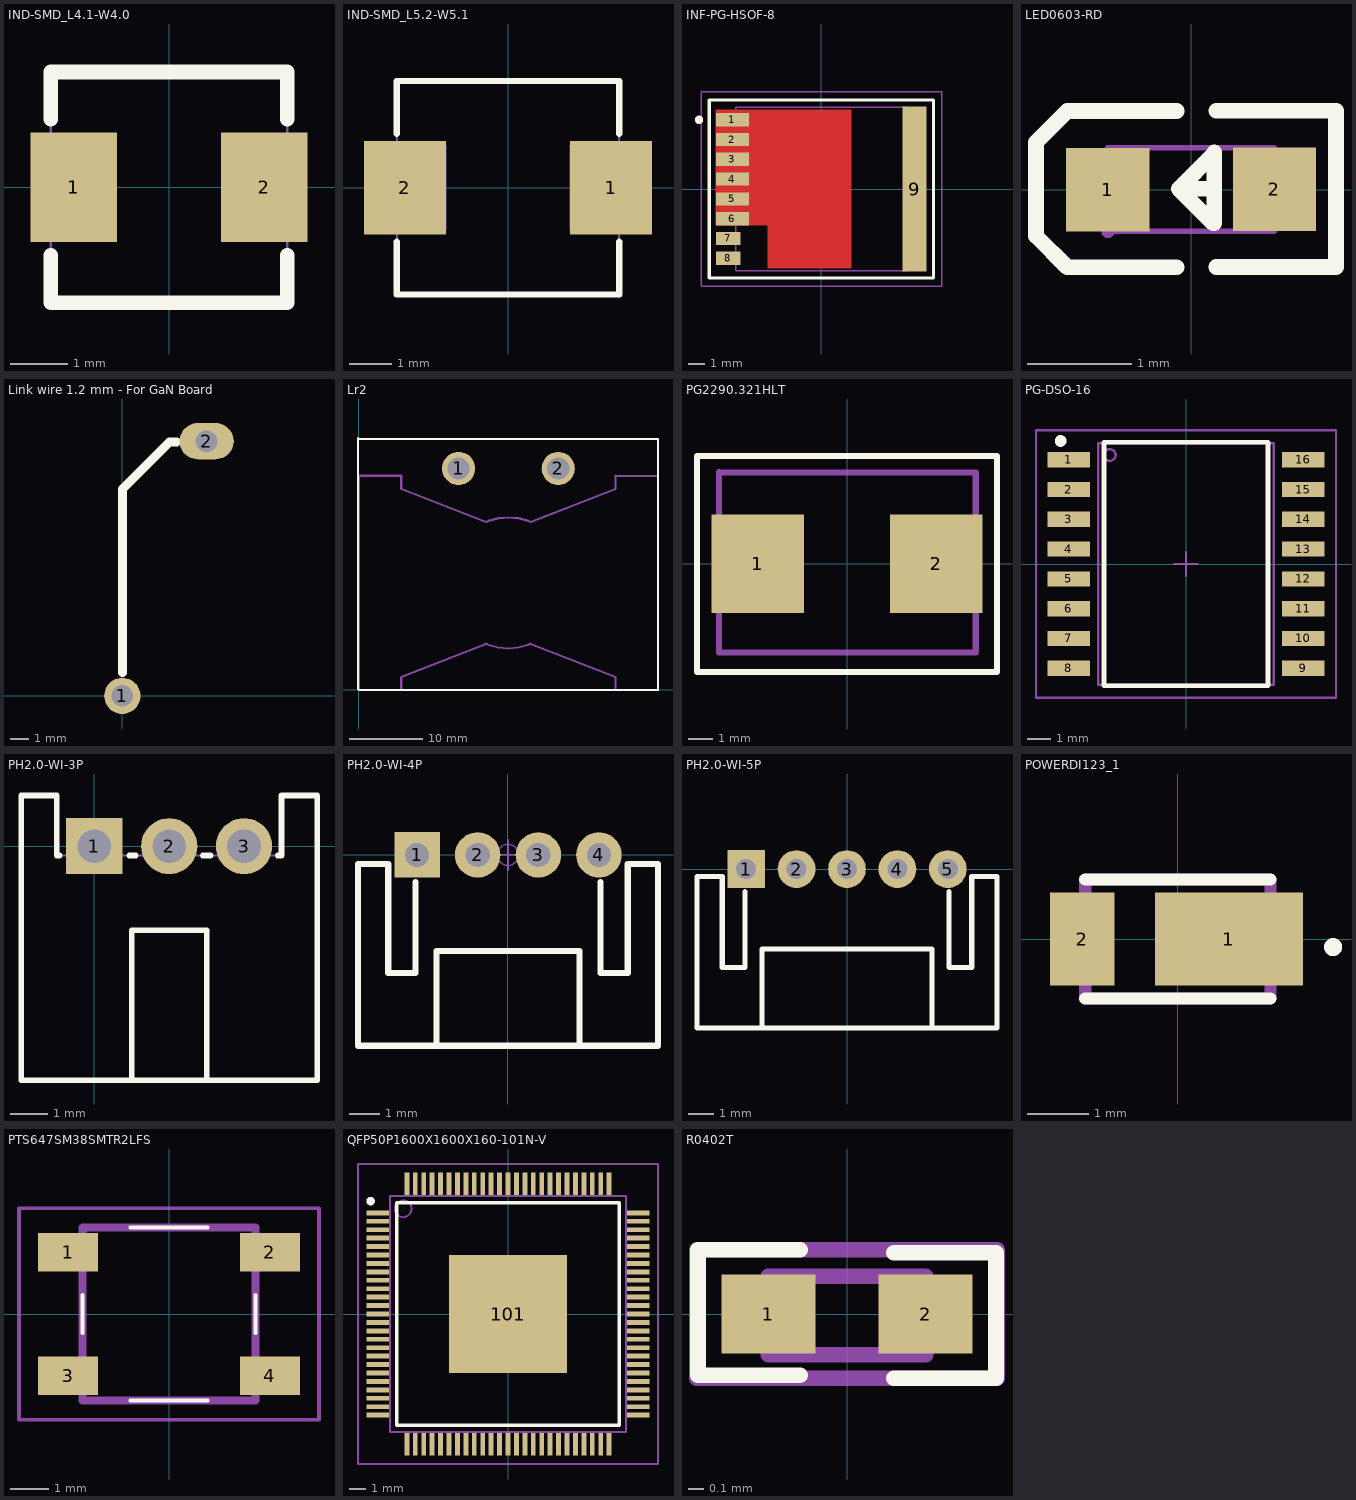
[diagram p0: the footprints below, top view; thin cyan lines are the x and y axes]
# Altium footprint library MISC82254-2.PcbLib: 93 footprints (part 3 of 6)
Each footprint in its own frame and in the unit in brackets; x right, y up, seen from the top. Pads: shape width x height; smd on the part's side, far side on the other; paste and mask are expansions set on the pad; w line width, h text height; cw(c..) or ccw(c..) is an arc to the next point about the centre after c.

## IND-SMD_L4.1-W4.0 [mm]
pads (2):
  rect 1.5x1.9 smd: 1(-1.651,0) 2(1.651,0)
Top Overlay:
  lines w0.254: -2.05,-1.181 -2.05,-2 2.05,-2 2.05,-1.181 ; -2.05,1.181 -2.05,1.999 1.831,1.999 2.05,2 2.05,1.181
Mechanical 15:
  region: -1.99,-2 -1.991,-1.976 -2.026,-1.942 -2.074,-1.942 -2.109,-1.976 -2.11,-2 -2.109,-2.024 -2.074,-2.058 -2.026,-2.058 -1.991,-2.024
  region: -2.05,0.8 -1.05,0.8 -1.05,-0.8 -2.05,-0.8
  region: 1.05,0.8 2.05,0.8 2.05,-0.8 1.05,-0.8
  lines w0.051: -2.05,-2 -2.05,2 2.05,2 2.05,-2 -2.05,-2
3D body "SPM4030T-1R5M-HZ.STEP": height 3, standoff 0, extent -2.1,-2 2.1,2

## IND-SMD_L5.2-W5.1 [mm]
pads (2):
  rect 1.924x2.2 smd: 1(2.412,0) 2(-2.412,0)
Top Overlay:
  lines w0.15: -2.6,-1.26 -2.6,-2.5 2.6,-2.5 2.6,-1.26 ; -2.6,1.26 -2.6,2.5 2.6,2.5 2.6,1.26
Mechanical 15:
  region: 2.66,-2.5 2.659,-2.476 2.624,-2.442 2.576,-2.442 2.541,-2.476 2.54,-2.5 2.541,-2.524 2.576,-2.558 2.624,-2.558 2.659,-2.524
  region: -2.6,-1 -2.6,1 -1.45,1 -1.45,-1
  region: 1.45,1 2.6,1 2.6,-1 1.45,-1
  lines w0.051: -2.6,-2.5 -2.6,2.5 2.6,2.5 2.6,-2.5 -2.6,-2.5
3D body "SPM5030T-3R3M-HZ.STEP": height 3, standoff 0, extent -2.6,-2.5 2.6,2.5

## INF-PG-HSOF-8 [mm] "Transistor; 9 pin, 10.375 mm L X 9.90 mm W X 2.40 mm H body"
height 2.4
pads (9):
  rect 2x0.8 smd paste-0.4 mask+0: 1(-5.4,4.2) 2(-5.4,3) 3(-5.4,1.8) 4(-5.4,0.6) 5(-5.4,-0.6) 6(-5.4,-1.8)
  rect 1.5x0.8 smd paste-0.05 mask+0: 7(-5.65,-3) 8(-5.65,-4.2)
  rect 1.45x10 smd paste-0.725 mask+0: 9(5.65,0)
Top Layer:
  region: -6.4,4.8 1.8,4.8 1.8,-4.8 -3.25,-4.8 -3.25,-2.2 -6.4,-2.2
Top Overlay:
  circle w0.25: c-7.427,4.2 r0.125
  lines w0.2: -6.8,-5.4 -6.8,5.4 6.8,5.4 6.8,-5.4 -6.8,-5.4
Top Paste:
  region: -0.75,0.2 -0.75,4.3 -1.55,4.3 -1.55,0.2
  region: 0.85,-0.2 1.65,-0.2 1.65,-4.7 0.85,-4.7
  region: 0.85,4.7 1.65,4.7 1.65,0.2 0.85,0.2
  region: -6.35,0.95 -4.55,0.95 -4.55,0.25 -6.35,0.25
  region: -6.35,2.15 -4.55,2.15 -4.55,1.45 -6.35,1.45
  region: -6.35,3.35 -4.55,3.35 -4.55,2.65 -6.35,2.65
  region: -6.35,4.55 -4.55,4.55 -4.55,3.85 -6.35,3.85
  region: -6.35,-0.25 -4.55,-0.25 -4.55,-0.95 -6.35,-0.95
  region: -6.35,-1.45 -4.55,-1.45 -4.55,-2.15 -6.35,-2.15
  region: 4.975,-1.25 6.325,-1.25 6.325,-2.75 4.975,-2.75
  region: 4.975,0.75 6.325,0.75 6.325,-0.75 4.975,-0.75
  region: 4.975,-3.25 6.325,-3.25 6.325,-4.75 4.975,-4.75
  region: 4.975,2.75 6.325,2.75 6.325,1.25 4.975,1.25
  region: -0.75,-4.3 -0.75,-0.2 -1.55,-0.2 -1.55,-4.3
  region: -0.35,4.7 0.45,4.7 0.45,0.2 -0.35,0.2
  region: 4.975,4.75 6.325,4.75 6.325,3.25 4.975,3.25
  region: -0.35,-0.2 0.45,-0.2 0.45,-4.7 -0.35,-4.7
  region: -1.95,-4.3 -1.95,-0.2 -2.75,-0.2 -2.75,-4.3
  region: -1.95,0.2 -1.95,4.3 -2.75,4.3 -2.75,0.2
  region: -3.15,-2.1 -3.15,-0.2 -3.95,-0.2 -3.95,-2.1
  region: -3.15,0.2 -3.15,4.3 -3.95,4.3 -3.95,0.2
Mechanical 3:
  text ".DESIGNATOR" at 0,0 h1.2
Mechanical 13:
  circle w0.1: c-4.328,4.166 r0.5
  lines w0.1: -5.197,-4.95 -5.197,4.95 5.178,4.95 5.178,-4.95 -5.197,-4.95
Mechanical 15:
  lines w0.1: -0.5,0 0.5,0 ; 0,-0.5 0,0.5 ; -7.3,-5.9 -7.3,5.9 7.3,5.9 7.3,-5.9 -7.3,-5.9
3D body "PG-HSOF-8.STEP": height 2.4, standoff 0, extent -5.798,-4.95 5.877,4.95

## LED0603-RD [mm]
pads (2):
  rect 0.8x0.8 smd: 1(-0.8,-0.003) 2(0.8,0.003)
Top Overlay:
  lines w0.15: -0.14,-0.746 -1.19,-0.746 -1.49,-0.446 -1.49,-0.346 -1.49,0.354 -1.49,0.454 -1.19,0.754 -0.14,0.754 ; 0.22,0.007 -0.12,0.007 ; 0.24,-0.744 1.39,-0.744 ; 0.24,0.757 1.39,0.757 1.39,-0.723 ; -0.12,0.007 0.21,-0.323 0.22,-0.323 0.22,0.357 0.22,0.347 -0.12,0.007
Mechanical 6:
  region: 0.529,0.068 1.069,0.068 1.069,-0.062 0.529,-0.062
  region: 0.735,-0.267 0.735,0.273 0.865,0.273 0.865,-0.267
  region: -1.07,0.062 -0.53,0.062 -0.53,-0.068 -1.07,-0.068
Mechanical 15:
  region: -0.74,-0.403 -0.741,-0.379 -0.775,-0.346 -0.824,-0.346 -0.858,-0.379 -0.859,-0.403 -0.858,-0.428 -0.824,-0.461 -0.775,-0.461 -0.741,-0.428
  region: 0.5,-0.396 0.5,0.404 0.8,0.404 0.8,-0.396
  region: -0.8,-0.403 -0.8,0.397 -0.5,0.397 -0.5,-0.403
  lines w0.051: -0.8,-0.4 -0.8,0.4 0.8,0.4 0.8,-0.4 -0.8,-0.4
3D body "SMLD12EN1WT86.stp": height 0.55, standoff 0, extent -0.927,-0.4 0.673,0.4

## Link wire 1.2 mm - For GaN Board [mm]
height 2
pads (2):
  round 2 hole 1.2: 1(0,0)
  oval 3x2 / inner oval 3x1.3 / far side oval 3x1.3 hole 1.2: 2(4.65,14.05)
Top Overlay:
  lines w0.5: 0,1.3 0,11.4 2.6,14 3,14
3D body: height 1.8, standoff 0.6, extent 4.056,13.403 5.25,14.598
3D body: height 1.2, standoff -3, extent -0.595,-0.599 0.6,0.599
3D body: height 1.2, standoff -3, extent 4.055,13.401 5.25,14.599
3D body: height 1.8, standoff 0.6, extent -0.594,-0.597 0.6,0.598
3D body: height 1.8, standoff 0.6, extent -0.599,0 0.599,11.5
3D body: height 1.8, standoff 0.6, extent 2.505,13.401 4.625,14.599
3D body: height 1.8, standoff 0.6, extent -0.597,10.65 3.352,14.599

## Lr2 [mm]
pads (2):
  round 4.5 hole 3: 1(13.5,30) 2(27,30)
Top Overlay:
  lines w0.254: -0.127,0.127 -0.127,34.127 ; -0.127,34 40.513,34 ; 0,0 40.513,0 40.513,33.951
Mechanical 13:
  lines w0.3: 5.74,0.009 5.74,1.709 ; 5.74,1.75 17.215,6.215 ; 5.742,27.225 17.217,22.76 17.217,22.733 17.591,22.908 18.896,23.257 20.242,23.375 21.588,23.257 22.893,22.908 23.267,22.733 23.267,22.76 34.742,27.225 ; 5.742,27.3 5.742,29 ; 5.75,0 0,0 0,29 5.75,29 ; 17.19,6.24 17.19,6.267 17.564,6.092 18.869,5.743 20.215,5.625 21.561,5.743 22.866,6.092 23.24,6.267 23.24,6.24 ; 23.265,6.215 34.74,1.75 ; 34.74,0.009 34.74,1.709 ; 34.742,0 40.492,0 ; 34.742,27.3 34.742,29 ; 34.744,28.991 40.494,28.991 40.494,-0.009
  text "PQ40磁芯" at 14.859,13.014 h3

## PCBComponent_1 [mm]

## PG2290.321HLT [mm]
pads (2):
  rect 3.85x4.1 smd: 1(-3.725,0) 2(3.725,0)
Top Overlay:
  lines w0.254: -6.25,-4.508 -6.25,4.492 ; -6.25,-4.5 6.25,-4.5 6.25,4.5 -6.25,4.5
Mechanical 1:
  lines w0.254: -5.334,-3.69 5.366,-3.69 5.366,3.81 -5.334,3.81 ; -5.334,-3.683 -5.334,3.817
3D body: height 12, standoff 0, extent -5.334,-3.683 5.334,3.81

## PG-DSO-16 [mm] "SOIC,1.27mm pitch;16 pin,7.50mm W X 10.30mm L X 2.65mm H body"
height 2.65
pads (16):
  rect 1.8x0.65 smd paste+0 mask+0: 1(-5,4.445) 2(-5,3.175) 3(-5,1.905) 4(-5,0.635) 5(-5,-0.635) 6(-5,-1.905) 7(-5,-3.175) 8(-5,-4.445) 9(5,-4.445) 10(5,-3.175) 11(5,-1.905) 12(5,-0.635) 13(5,0.635) 14(5,1.905) 15(5,3.175) 16(5,4.445)
Top Overlay:
  circle w0.25: c-5.35,5.25 r0.125
  lines w0.2: -3.5,-5.2 -3.5,5.2 3.5,5.2 3.5,-5.2 -3.5,-5.2
Mechanical 3:
  text ".DESIGNATOR" at 0,0 h1.2
Mechanical 13:
  circle w0.1: c-3.25,4.65 r0.25
  lines w0.1: -3.75,-5.15 -3.75,5.15 3.75,5.15 3.75,-5.15 -3.75,-5.15
Mechanical 15:
  lines w0.1: -0.5,0 0.5,0 ; 0,-0.5 0,0.5 ; -6.4,-5.7 -6.4,5.7 6.4,5.7 6.4,-5.7 -6.4,-5.7
3D body "DSO-16-30.stp": height 2.66, standoff 0, extent -5.15,-5.15 5.15,5.15

## PH2.0-WI-3P [mm] "长：7.9mm，宽：6mm，高：4.7mm"
height 10
pads (3):
  rect 1.5x1.5 hole 0.9: 1(0,0)
  round 1.5 hole 0.9: 2(2,0) 3(4,0)
Top Overlay:
  lines w0.152: -0.93,-0.25 -1,-0.25 -1,1.35 -1.95,1.35 -1.95,-6.25 5.95,-6.25 5.95,1.35 5,1.35 5,-0.25 4.896,-0.25 ; 0.93,-0.25 1.104,-0.25 ; 1.001,-6.25 1.001,-2.25 3,-2.25 3,-6.25 ; 2.896,-0.25 3.104,-0.25
Mechanical 6:
  region: -2,-5.4 -2,-6.2 -1.9,-6.3 5.9,-6.3 6,-6.2 6,-5.6 5.9,-5.6 5.9,-6.2 -1.9,-6.2 -1.9,-5.4
Mechanical 15:
  region: -1.89,-6.25 -1.89,-6.225 -1.925,-6.19 -1.975,-6.19 -2.01,-6.225 -2.01,-6.25 -2.01,-6.275 -1.975,-6.31 -1.925,-6.31 -1.89,-6.275
  region: 3.75,0.25 4.25,0.25 4.25,-0.25 3.75,-0.25
  region: 1.75,0.25 2.25,0.25 2.25,-0.25 1.75,-0.25
  region: -0.25,0.25 0.25,0.25 0.25,-0.25 -0.25,-0.25
  region: 4.25,0.25 4.25,-0.26 3.75,-0.26 3.75,0.24 3.75,0.25
  region: 2.25,0.25 2.25,-0.26 1.75,-0.26 1.75,0.24 1.75,0.25
  region: 0.25,0.25 0.25,-0.26 -0.25,-0.26 -0.25,0.24 -0.25,0.25
  lines w0.051: -1.95,-6.25 5.95,-6.25 5.95,1.35 5,1.35 5,-0.25 2,-0.25 -1,-0.25 -1,1.35 -1.95,1.35 -1.95,-6.25
3D body "PH2.0-WI-3P.STEP": height 4.75, standoff -2.65, extent -1.95,-6.3 5.95,0.3

## PH2.0-WI-4P [mm] "长：9.9mm，宽：6mm，高：4.7mm"
height 10
pads (4):
  rect 1.5x1.5 hole 0.8: 1(-3,0)
  round 1.5 hole 0.8: 2(-1,0) 3(1,0) 4(3,0)
Top Overlay:
  lines w0.203: -3.05,-0.9 -3.05,-3.9 -3.95,-3.9 -3.95,-3.3 -3.95,-0.3 -4,-0.3 -4.95,-0.3 -4.95,-6.3 4.95,-6.3 4.95,-0.3 4,-0.3 3.95,-0.3 3.95,-3.3 3.95,-3.9 3.05,-3.9 3.05,-0.9 ; -2.365,-6.215 -2.365,-3.175 2.365,-3.175 2.365,-6.215
Mechanical 15:
  circle w0.05: c0,0 r0.35
  lines w0.05: -0.5,0 0.5,0 ; 0,-0.5 0,0.5
3D body "PH2.0-WI-4P.STEP": height 4.75, standoff -2.65, extent -4.95,-6.3 4.95,0.3

## PH2.0-WI-5P [mm] "长：11.9mm，宽：6mm，高：4.7mm"
height 10
pads (5):
  rect 1.5x1.5 hole 0.8: 1(-4,0)
  round 1.5 hole 0.8: 2(-2,0) 3(0,0) 4(2,0) 5(4,0)
Top Overlay:
  lines w0.203: -4.05,-0.9 -4.05,-3.9 -4.95,-3.9 -4.95,-3.3 -4.95,-0.3 -5,-0.3 -5.95,-0.3 -5.95,-6.3 5.95,-6.3 5.95,-0.3 5,-0.3 4.95,-0.3 4.95,-3.3 4.95,-3.9 4.05,-3.9 4.05,-0.9 ; -3.365,-6.215 -3.365,-3.175 3.365,-3.175 3.365,-6.215
Mechanical 15:
  circle w0.05: c0,0 r0.35
  lines w0.05: -0.5,0 0.5,0 ; 0,-0.5 0,0.5
3D body "PH2.0-WI-5P.STEP": height 4.75, standoff -2.65, extent -5.95,-6.3 5.95,0.3

## POWERDI123_1 [mm]
pads (2):
  rect 2.4x1.5 smd: 1(0.825,0)
  rect 1.05x1.5 smd: 2(-1.55,0)
Top Overlay:
  circle w0.2: c2.515,-0.131 r0.046
  lines w0.2: -1.5,-0.965 1.5,-0.965 ; -1.5,0.965 1.5,0.965
Mechanical 13:
  lines w0.2: -1.5,-0.965 1.5,-0.965 1.5,0.965 -1.5,0.965 -1.5,-0.965
3D body "DFLS1100-7.stp": height 0.98, standoff 0, extent -1.85,-0.89 1.85,0.89

## PTS647SM38SMTR2LFS [mm]
pads (4):
  rect 1.55x1 smd: 1(-2.625,1.6) 2(2.625,1.6) 3(-2.625,-1.6) 4(2.625,-1.6)
Top Overlay:
  lines w0.1: -2.25,-0.5 -2.25,0.5 ; -1,-2.25 1,-2.25 ; -1,2.25 1,2.25 ; 2.25,-0.5 2.25,0.5
Mechanical 13:
  lines w0.2: -2.25,-2.25 -2.25,2.25 2.25,2.25 2.25,-2.25 -2.25,-2.25
Mechanical 15:
  lines w0.1: -3.9,-2.75 -3.9,2.75 3.9,2.75 3.9,-2.75 -3.9,-2.75
3D body "PTS647SM38SMTR2LFS.stp": height 3.8, standoff 0, extent -3.25,-2.25 3.25,2.25

## QFP50P1600X1600X160-101N-V [mm] "QFP,0.50mm pitch,square;100 pin,14.00mm L X 14.00mm W X 1.60mm H body (w/thermal tab)"
height 1.6
pads (101):
  rect 1.35x0.29 smd paste+0 mask+0: 1(-7.725,6) 2(-7.725,5.5) 3(-7.725,5) 4(-7.725,4.5) 5(-7.725,4) 6(-7.725,3.5) 7(-7.725,3) 8(-7.725,2.5) 9(-7.725,2) 10(-7.725,1.5) 11(-7.725,1) 12(-7.725,0.5) 13(-7.725,0) 14(-7.725,-0.5) 15(-7.725,-1) 16(-7.725,-1.5) 17(-7.725,-2) 18(-7.725,-2.5) 19(-7.725,-3) 20(-7.725,-3.5) 21(-7.725,-4) 22(-7.725,-4.5) 23(-7.725,-5) 24(-7.725,-5.5) 25(-7.725,-6) 51(7.725,-6) 52(7.725,-5.5) 53(7.725,-5) 54(7.725,-4.5) 55(7.725,-4) 56(7.725,-3.5) 57(7.725,-3) 58(7.725,-2.5) 59(7.725,-2) 60(7.725,-1.5) 61(7.725,-1) 62(7.725,-0.5) 63(7.725,0) 64(7.725,0.5) 65(7.725,1) 66(7.725,1.5) 67(7.725,2) 68(7.725,2.5) 69(7.725,3) 70(7.725,3.5) 71(7.725,4) 72(7.725,4.5) 73(7.725,5) 74(7.725,5.5) 75(7.725,6)
  rect 0.29x1.35 smd paste+0 mask+0: 26(-6,-7.725) 27(-5.5,-7.725) 28(-5,-7.725) 29(-4.5,-7.725) 30(-4,-7.725) 31(-3.5,-7.725) 32(-3,-7.725) 33(-2.5,-7.725) 34(-2,-7.725) 35(-1.5,-7.725) 36(-1,-7.725) 37(-0.5,-7.725) 38(0,-7.725) 39(0.5,-7.725) 40(1,-7.725) 41(1.5,-7.725) 42(2,-7.725) 43(2.5,-7.725) 44(3,-7.725) 45(3.5,-7.725) 46(4,-7.725) 47(4.5,-7.725) 48(5,-7.725) 49(5.5,-7.725) 50(6,-7.725) 76(6,7.725) 77(5.5,7.725) 78(5,7.725) 79(4.5,7.725) 80(4,7.725) 81(3.5,7.725) 82(3,7.725) 83(2.5,7.725) 84(2,7.725) 85(1.5,7.725) 86(1,7.725) 87(0.5,7.725) 88(0,7.725) 89(-0.5,7.725) 90(-1,7.725) 91(-1.5,7.725) 92(-2,7.725) 93(-2.5,7.725) 94(-3,7.725) 95(-3.5,7.725) 96(-4,7.725) 97(-4.5,7.725) 98(-5,7.725) 99(-5.5,7.725) 100(-6,7.725)
  rect 7x7 smd paste+0 mask+0: 101(0,0)
Top Overlay:
  circle w0.25: c-8.153,6.695 r0.125
  lines w0.2: -6.6,-6.6 -6.6,6.6 6.6,6.6 6.6,-6.6 -6.6,-6.6
Mechanical 3:
  text ".DESIGNATOR" at 0,0 h1.2
Mechanical 13:
  circle w0.1: c-6.223,6.248 r0.5
  lines w0.1: -7,-7 -7,7 7,7 7,-7 -7,-7
Mechanical 15:
  lines w0.1: -0.5,0 0.5,0 ; 0,-0.5 0,0.5 ; -8.9,-8.9 -8.9,8.9 8.9,8.9 8.9,-8.9 -8.9,-8.9
3D body "PG-LQFP-100-25.STEP": height 1.61, standoff 0, extent -8,-8 8,8

## R0402T [mm]
pads (2):
  rect 0.6x0.5 smd mask+0.05: 1(-0.5,0) 2(0.5,0)
Top Overlay:
  lines w0.1: -0.298,-0.39 -0.949,-0.39 -0.949,0.41 -0.298,0.41 ; 0.298,-0.41 0.949,-0.41 0.949,0.39 0.298,0.39
Mechanical 13:
  lines w0.1: -0.5,-0.26 0.5,-0.26 0.5,0.24 -0.5,0.24 -0.5,-0.26
Mechanical 15:
  lines w0.1: -0.955,-0.41 0.955,-0.41 0.955,0.39 ; -0.955,-0.39 -0.955,0.41 0.955,0.41
3D body "CPF0402B100KE.stp": height 0.35, standoff 0, extent -0.5,-0.25 0.5,0.25